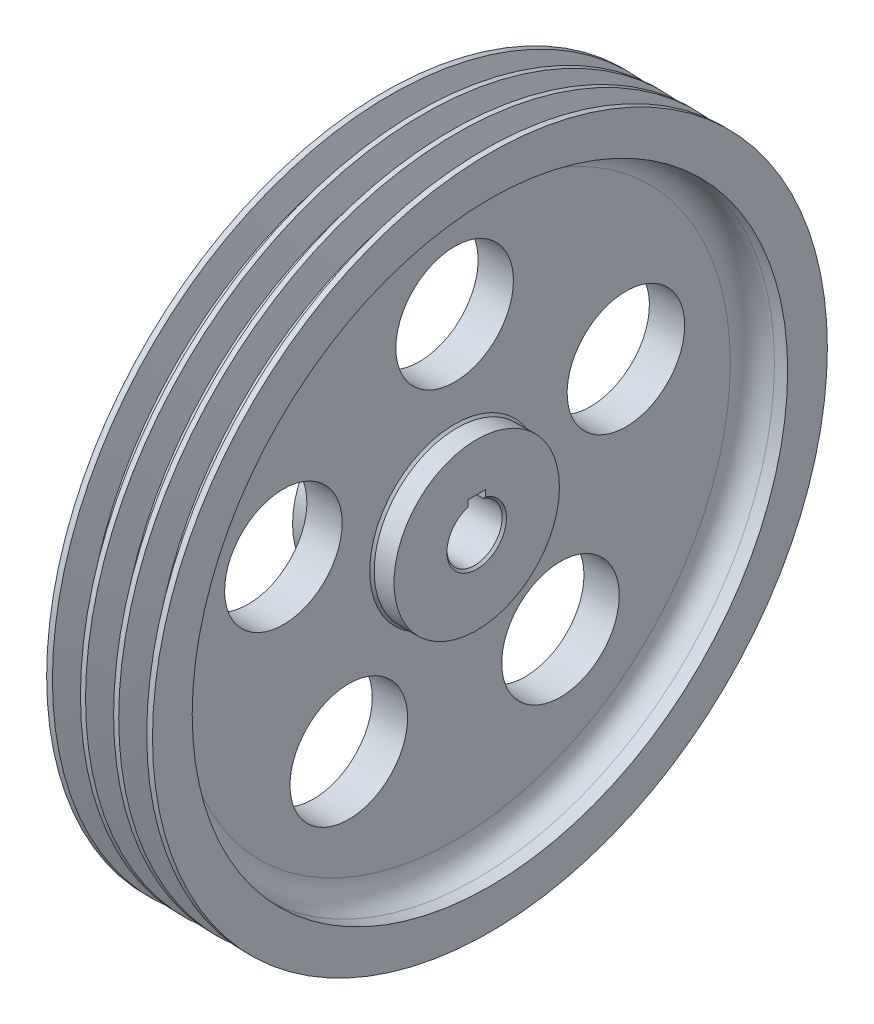
from build123d import *

# Parameters (mm, degrees)
SKETCH8_R           = 37.5
SKETCH8_R_2         = 12.5
BOSS_EXTRUDE2_DEPTH = 4
CUT_EXTRUDE5_REACH  = 224.535
SKETCH9_W           = 8
SKETCH9_H           = 6.6
CUT_EXTRUDE6_START  = -16
SKETCH10_R          = 135
SKETCH10_R_2        = 37.5
CUT_EXTRUDE6_DEPTH  = 16
SKETCH11_R          = 135
SKETCH11_R_2        = 37.5
CUT_EXTRUDE7_DEPTH  = 16
FILLET1_R           = 10
CHAMFER1_SIZE       = 1
SKETCH13_R          = 37.5
CUT_EXTRUDE9_DEPTH  = 6
CHAMFER2_SIZE       = 1
CUT_EXTRUDE8_REACH  = 220.728
SKETCH12_R          = 26.65
CIRPATTERN1_COUNT   = 5


with BuildPart() as part:
    # Sketch1 → Revolve1 (revolve)
    with BuildSketch(Plane.XY, mode=Mode.PRIVATE) as revolve1_sk:
        Polygon((6.128194326, 141.5), (2.61229149, 153), (0, 153), (0, 12.5), (48, 12.5), (48, 153), (45.38770851, 153), (41.871805674, 141.5), (36.191805674, 141.5), (32.675902837, 153), (30.355902837, 153), (26.84, 141.5), (21.16, 141.5), (17.644097163, 153), (15.324097163, 153), (11.808194326, 141.5), align=None)
    revolve(revolve1_sk.sketch.rotate(Axis((0, 0, 0), (1, 0, 0)), 270), axis=Axis((0, 0, 0), (1, 0, 0)))

    # Sketch8 → Boss-Extrude2 (add)
    with BuildSketch(Plane.ZY):
        Circle(SKETCH8_R)
        with Locations(Location((0, 0, 0), (0, 0, 180))):
            Circle(SKETCH8_R_2, mode=Mode.SUBTRACT)
    extrude(amount=BOSS_EXTRUDE2_DEPTH)

    # Sketch9 → Cut-Extrude5 (cut, up to next)
    with BuildSketch(Plane.ZY.offset(4), mode=Mode.PRIVATE) as cut_extrude5_sk1:
        with Locations((0, 12.5)):
            Rectangle(SKETCH9_W, SKETCH9_H)
    cut_extrude5_tool1 = extrude(cut_extrude5_sk1.sketch, amount=-CUT_EXTRUDE5_REACH, mode=Mode.PRIVATE) & part.part
    add(cut_extrude5_tool1.solids().sort_by_distance((-4, 12.5, 0))[0], mode=Mode.SUBTRACT)

    # Sketch10 → Cut-Extrude6 (cut)
    with BuildSketch(Plane.ZY.offset(CUT_EXTRUDE6_START)):
        Circle(SKETCH10_R)
        Circle(SKETCH10_R_2, mode=Mode.SUBTRACT)
    extrude(amount=CUT_EXTRUDE6_DEPTH, mode=Mode.SUBTRACT)

    # Sketch11 → Cut-Extrude7 (cut)
    with BuildSketch(Plane(origin=(48, 0, 0), x_dir=(0, 0, -1), z_dir=(1, 0, 0))):
        with Locations(Location((0, 0, 0), (0, 0, 180))):
            Circle(SKETCH11_R)
        with Locations(Location((0, 0, 0), (0, 0, 180))):
            Circle(SKETCH11_R_2, mode=Mode.SUBTRACT)
    extrude(amount=-CUT_EXTRUDE7_DEPTH, mode=Mode.SUBTRACT)

    # Fillet1
    fillet1_edges = [part.edges().sort_by_distance(p)[0] for p in [
        (16, 0, -135),
        (32, 0, -135),
    ]]
    fillet(fillet1_edges, radius=FILLET1_R)

    # Chamfer1
    chamfer1_edges = [part.edges().sort_by_distance(p)[0] for p in [
        (16, 0, -37.5),
        (32, 0, -37.5),
    ]]
    chamfer(chamfer1_edges, length=CHAMFER1_SIZE)

    # Sketch13 → Cut-Extrude9 (cut)
    with BuildSketch(Plane(origin=(48, 0, 0), x_dir=(0, 0, -1), z_dir=(1, 0, 0))):
        Circle(SKETCH13_R)
    extrude(amount=-CUT_EXTRUDE9_DEPTH, mode=Mode.SUBTRACT)

    # Chamfer2
    chamfer2_edges = [part.edges().sort_by_distance(p)[0] for p in [
        (-4, -12.5, 0),
        (42, -12.5, 0),
    ]]
    chamfer(chamfer2_edges, length=CHAMFER2_SIZE)

    # Sketch12 → Cut-Extrude8 (cut, up to next)
    with BuildSketch(Plane.ZY.offset(-16), mode=Mode.PRIVATE) as cut_extrude8_sk1:
        with Locations((0, 81.65)):
            Circle(SKETCH12_R)
    cut_extrude8_tool1 = extrude(cut_extrude8_sk1.sketch, amount=-CUT_EXTRUDE8_REACH, mode=Mode.PRIVATE) & part.part
    cut_extrude8 = cut_extrude8_tool1.solids().sort_by_distance((16, 81.65, 0))[0]
    add(cut_extrude8, mode=Mode.SUBTRACT)

    # CirPattern1: Cut-Extrude8 ×5 about axis
    cirpattern1_axis = Axis((0, 0, 0), (1, 0, 0))
    for i in range(1, CIRPATTERN1_COUNT):
        add(cut_extrude8.rotate(cirpattern1_axis, i * 360 / CIRPATTERN1_COUNT), mode=Mode.SUBTRACT)


solid = part.part
